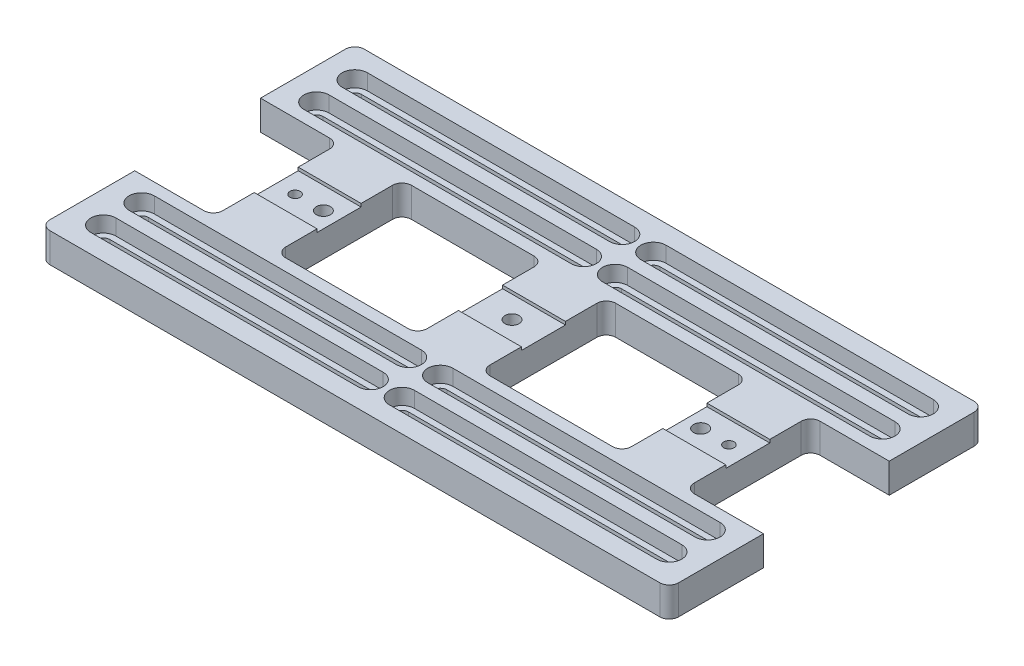
SolidWorks part; units mm, degrees
ref_plane "Front Plane" through (0, 0, 0) normal (0, 0, 1) x (1, 0, 0)
ref_plane "Top Plane" through (0, 0, 0) normal (0, 1, 0) x (1, 0, 0)
ref_plane "Right Plane" through (0, 0, 0) normal (1, 0, 0) x (0, 0, -1)
sketch "Sketch1" plane through (0, 0, 0) normal (0, 1, 0) x (1, 0, 0)
  line L1 (100, -50) -> (-100, -50)
  line L2 (100, -50) -> (100, 50)
  line L3 (100, 50) -> (-100, 50)
  line L4 (-100, -50) -> (-100, 50)
  line L5 (100, -50) -> (-100, 50) construction
  line L6 (100, 50) -> (-100, -50) construction
  point P0 (0, 0)
  dimension "D1" = 200
  dimension "D2" = 100
extrude "Boss-Extrude1" add sketch "Sketch1" along normal mid plane 9.4
fillet "Fillet1" radius 3 4 edges at (-100, 0, -50) (-100, 0, 50) (100, 0, -50) (100, 0, 50)
sketch "Sketch2" plane through (0, 4.7, 0) normal (0, 1, 0) x (1, 0, 0)
  line L0 (100, -47) -> (100, 47) construction
  line L1 (125, -20) -> (75, -20)
  line L2 (125, -20) -> (125, 20)
  line L3 (125, 20) -> (75, 20)
  line L4 (75, -20) -> (75, 20)
  line L5 (125, -20) -> (75, 20) construction
  line L6 (125, 20) -> (75, -20) construction
  point P0 (100, 0)
  dimension "D1" = 40
  dimension "D2" = 25
extrude "Cut-Extrude1" cut sketch "Sketch2" against normal through all
mirror "Mirror1" about plane through (0, 0, 0) normal (1, 0, 0) of "Cut-Extrude1"
sketch "Sketch3" plane through (0, 4.7, 0) normal (0, 1, 0) x (1, 0, 0)
  line L0 (-75, 20) -> (-75, -20) construction
  line L1 (-10, -20) -> (-55, -20)
  line L2 (-10, -20) -> (-10, 20)
  line L3 (-10, 20) -> (-55, 20)
  line L4 (-55, -20) -> (-55, 20)
  line L5 (-10, -20) -> (-55, 20) construction
  line L6 (-10, 20) -> (-55, -20) construction
  point P0 (-32.5, 0)
  dimension "D1" = 20
  dimension "D2" = 40
  dimension "D3" = 45
extrude "Cut-Extrude2" cut sketch "Sketch3" against normal through all
fillet "Fillet2" radius 3 4 edges at (75, 0, 20) (75, 0, -20) (-75, 0, 20) (-75, 0, -20)
fillet "Fillet3" radius 3 4 edges at (-10, 0, -20) (-10, 0, 20) (-55, 0, 20) (-55, 0, -20)
mirror "Mirror2" about plane through (0, 0, 0) normal (1, 0, 0) of "Fillet3", "Cut-Extrude2"
sketch "Sketch4" plane through (0, 4.7, 0) normal (0, 1, 0) x (1, 0, 0)
  line L0 (-90, -40) -> (-5, -40) construction
  line L1 (-90, -36) -> (-5, -36)
  line L2 (-90, -44) -> (-5, -44)
  line L3 (-100, -20) -> (-100, -47) construction
  line L4 (-90, -31.8) -> (-5, -31.8)
  line L5 (-97, -50) -> (97, -50) construction
  line L6 (-90, -23.8) -> (-5, -23.8)
  line L7 (-90, -27.8) -> (-5, -27.8) construction
  arc A0 (-90, -36) -> (-90, -44) centre (-90, -40) ccw
  arc A1 (-5, -44) -> (-5, -36) centre (-5, -40) ccw
  arc A2 (-90, -23.8) -> (-90, -31.8) centre (-90, -27.8) ccw
  arc A3 (-5, -31.8) -> (-5, -23.8) centre (-5, -27.8) ccw
  point P2 (-47.5, -40)
  point P15 (-47.5, -27.8)
  dimension "D4" = 4
  dimension "D1" = 10
  dimension "D2" = 85
  dimension "D3" = 6
  dimension "D5" = 2
extrude "Cut-Extrude3" cut sketch "Sketch4" against normal blind 5
sketch "Sketch5" plane through (0, -0.3, 0) normal (0, 1, 0) x (1, 0, 0)
  line L0 (-90, -27.8) -> (-5, -27.8) construction
  line L1 (-90, -25.7) -> (-5, -25.7)
  line L2 (-90, -29.9) -> (-5, -29.9)
  line L3 (-90, -40) -> (-5, -40) construction
  line L4 (-90, -37.9) -> (-5, -37.9)
  line L5 (-90, -42.1) -> (-5, -42.1)
  arc A0 (-90, -25.7) -> (-90, -29.9) centre (-90, -27.8) ccw
  arc A1 (-5, -29.9) -> (-5, -25.7) centre (-5, -27.8) ccw
  arc A2 (-90, -37.9) -> (-90, -42.1) centre (-90, -40) ccw
  arc A3 (-5, -42.1) -> (-5, -37.9) centre (-5, -40) ccw
  point P2 (-47.5, -27.8)
  point P11 (-47.5, -40)
  dimension "D1" = 2.1
  dimension "D2" = 2.1
extrude "Cut-Extrude4" cut sketch "Sketch5" against normal through all
mirror "Mirror3" about plane through (0, 0, 0) normal (1, 0, 0) of "Cut-Extrude4", "Cut-Extrude3" second plane through (0, 0, 0) second plane normal (0, 0, 1)
sketch "Sketch6" plane through (0, 4.7, 0) normal (0, 1, 0) x (1, 0, 0)
  line L0 (-75, 17) -> (-75, -17) construction
  line L1 (75, -7) -> (-75, -7)
  line L2 (75, -7) -> (75, 7)
  line L3 (75, 7) -> (-75, 7)
  line L4 (-75, -7) -> (-75, 7)
  line L5 (75, -7) -> (-75, 7) construction
  line L6 (75, 7) -> (-75, -7) construction
  point P0 (0, 0)
  dimension "D1" = 14
extrude "Cut-Extrude5" cut sketch "Sketch6" against normal blind 1
hole_wizard "M4 Tapped Hole1" positions "Sketch7" profile "Sketch8" tap size "M4" standard "GB"
sketch "Sketch7" plane through (0, -4.7, 0) normal (0, -1, 0) x (-1, 0, 0)
  line L0 (-55, 0) -> (-75, 0) construction
  line L1 (-55, 17) -> (-55, -17) construction
  line L2 (-75, 17) -> (-75, -17) construction
  line L11 (0, 0) -> (0, -64.5845) construction
  point P0 (-69, 0)
  point P15 (-69, 0)
  point P42 (69, 0)
  dimension "D1" = 6
sketch "Sketch8" plane through (69, -4.7, 0) normal (1, 0, 0) x (0, 0, -1)
  line L0 (0, 0) -> (0, 12.4914)
  line L1 (0, 12.4914) -> (1.65, 11.5)
  line L2 (1.65, 11.5) -> (1.65, 0)
  line L5 (1.65, 0) -> (0, 0)
  line L10 (0, 12.4914) -> (-1.65, 11.5) construction
  line L11 (0, -6.35) -> (0, 107.95) construction
  dimension "螺纹孔钻头直径" = 3.3
  dimension "螺纹孔钻头深度" = 11.5
  dimension "导头角度" = 118
cosmetic thread "HoleThreadLine1" parameters "D1"=8, "D2"=4
cosmetic thread "HoleThreadLine2" parameters "D1"=8, "D2"=4
cosmetic thread "HoleThreadLine3" parameters "D1"=8, "D2"=4
hole_wizard "CBORE for M4 Hexagon socket head cap screws1" positions "Sketch9" profile "Sketch10" counterbore size "M4" standard "GB"
sketch "Sketch9" plane through (0, -4.7, 0) normal (0, -1, 0) x (-1, 0, 0)
  line L0 (-55, 17) -> (-55, -17) construction
  line L4 (0, 0) -> (0, 83.2862) construction
  line L6 (0, 0) -> (-60, 0) construction
  point P0 (-60, 0)
  point P14 (0, 0)
  point P18 (60, 0)
  point P21 (0, 0)
  dimension "D1" = 5
sketch "Sketch10" plane through (60, -4.7, 0) normal (1, 0, 0) x (0, 0, -1)
  line L0 (0, 0) -> (0, 12.8519)
  line L1 (0, 12.8519) -> (2.25, 11.5)
  line L2 (2.25, 11.5) -> (2.25, 4.6)
  line L3 (2.25, 4.6) -> (4, 4.6)
  line L4 (4, 4.6) -> (4, 0)
  line L5 (4, 0) -> (0, 0)
  line L10 (0, 12.8519) -> (-2.25, 11.5) construction
  line L11 (0, -6.35) -> (0, 107.95) construction
  dimension "孔直径" = 4.5
  dimension "孔深度" = 11.5
  dimension "柱形沉头孔直径" = 8
  dimension "柱形沉头孔深度" = 4.6
  dimension "导头角度" = 118
equation "\"1\"= \"代号代号\""
equation "\"2\"= \"名称代号\""
